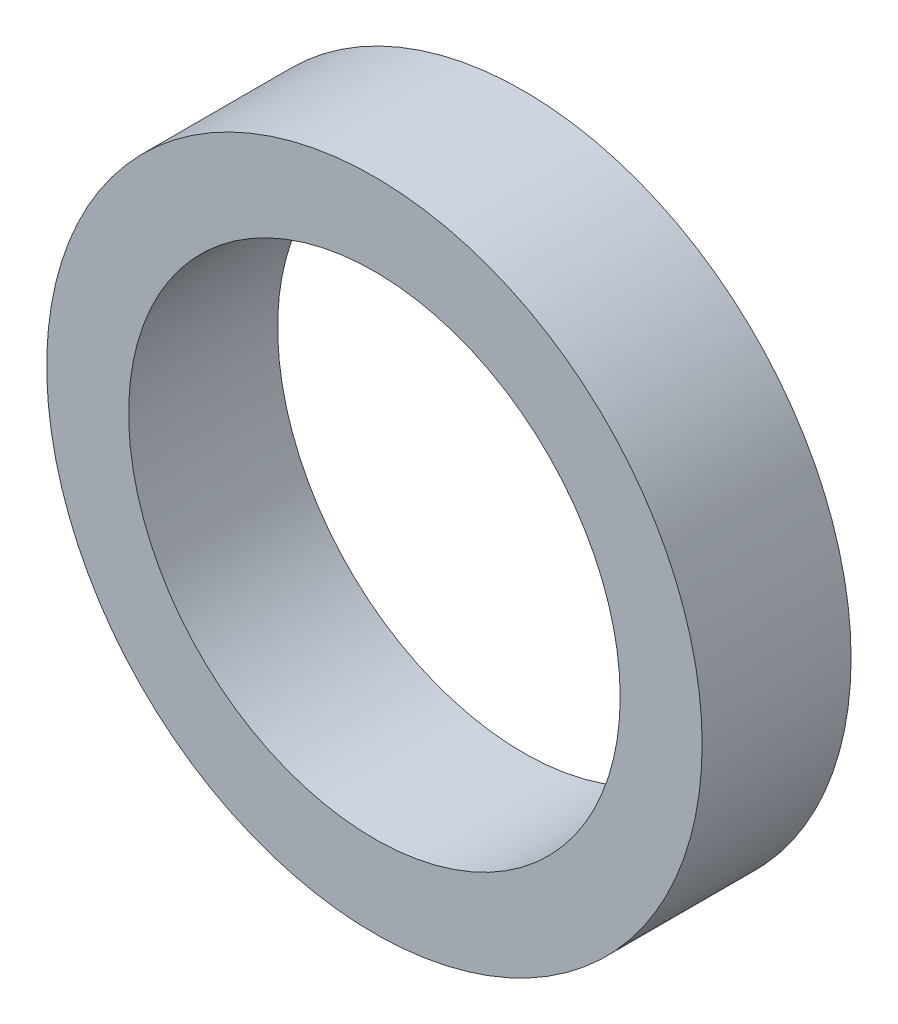
SolidWorks part; units mm, degrees
ref_plane "前视基准面" through (0, 0, 0) normal (0, 0, 1) x (1, 0, 0)
ref_plane "上视基准面" through (0, 0, 0) normal (0, 1, 0) x (1, 0, 0)
ref_plane "右视基准面" through (0, 0, 0) normal (1, 0, 0) x (0, 0, -1)
sketch "草图1" plane through (0, 0, 0) normal (0, 0, 1) x (1, 0, 0)
  circle A0 centre (0, 0) radius 8.25
  circle A1 centre (0, 0) radius 11
  dimension "D1" = 16.5
  dimension "D2" = 22
extrude "凸台-拉伸1" add sketch "草图1" along normal mid plane 5
